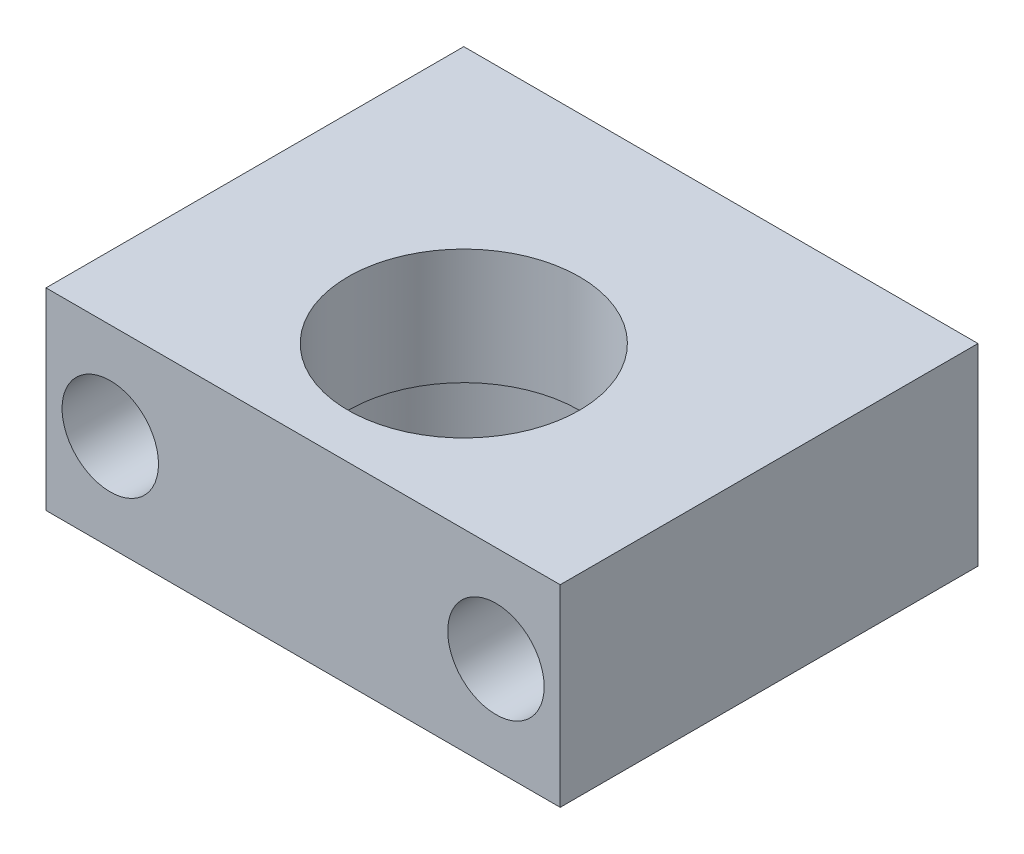
SolidWorks part; units mm, degrees
material "A6061"
ref_plane "前基準面" through (0, 0, 0) normal (0, 0, 1) x (1, 0, 0)
ref_plane "上基準面" through (0, 0, 0) normal (0, 1, 0) x (1, 0, 0)
ref_plane "右基準面" through (0, 0, 0) normal (1, 0, 0) x (0, 0, -1)
sketch "草图1" plane through (0, 0, 0) normal (0, 1, 0) x (1, 0, 0)
  line L1 (-225, -32.5) -> (225, -32.5)
  line L2 (-225, -32.5) -> (-225, 32.5)
  line L3 (-225, 32.5) -> (225, 32.5)
  line L4 (225, -32.5) -> (225, 32.5)
  line L5 (-225, -32.5) -> (225, 32.5) construction
  line L6 (-225, 32.5) -> (225, -32.5) construction
  point P0 (0, 0)
  dimension "D1" = 450
  dimension "D2" = 65
extrude "凸台-拉伸1" add sketch "草图1" along normal mid plane 30
chamfer "倒角1" distance 2 angle 45 2 edges at (225, 0, 32.5) (-225, 0, 32.5)
sketch "草图2" plane through (0, 15, 0) normal (0, 1, 0) x (1, 0, 0)
  line L0 (0, 83.4721) -> (0, 0) construction
  circle A0 centre (-200, 0) radius 10
  circle A1 centre (200, 0) radius 10
  dimension "D1" = 20
  dimension "D2" = 400
extrude "切除-拉伸1" cut sketch "草图2" against normal up to surface (30 mm away) up to face at (0, -15, 10.1667)
sketch "草图3" plane through (0, 15, 0) normal (0, 1, 0) x (1, 0, 0)
  line L0 (-225, 0) -> (-182, 0) construction
  line L2 (-225, 1) -> (-182, 1)
  line L3 (-225, -1) -> (-182, -1)
  line L4 (0, 108.9264) -> (0, 0) construction
  line L5 (225, 0) -> (182, 0) construction
  line L6 (225, 1) -> (182, 1)
  line L7 (225, -1) -> (182, -1)
  line L8 (-225, 32.5) -> (-225, -30.5) construction
  arc A0 (-225, 1) -> (-225, -1) centre (-225, 0) ccw
  arc A1 (-182, -1) -> (-182, 1) centre (-182, 0) ccw
  circle A2 centre (-200, 0) radius 10 construction
  arc A3 (225, 1) -> (225, -1) centre (225, 0) cw
  arc A4 (182, -1) -> (182, 1) centre (182, 0) cw
  point P2 (-200, 0)
  point P4 (-203.5, 0)
  point P16 (203.5, 0)
  dimension "D1" = 18
  dimension "D2" = 2
extrude "切除-拉伸2" cut sketch "草图3" against normal up to surface (30 mm away) up to face at (-200, -15, -10)
sketch "草图4" plane through (0, -15, 0) normal (0, 1, 0) x (1, 0, 0)
  line L0 (0, 70.3948) -> (0, 0) construction
  line L1 (225, 32.5) -> (-225, 32.5) construction
  circle A0 centre (0, -7.5) radius 21
  dimension "D1" = 42
  dimension "D2" = 40
extrude "切除-拉伸3" cut sketch "草图4" along normal blind 12
sketch "草图5" plane through (0, -3, 0) normal (0, -1, 0) x (-1, 0, 0)
  circle A0 centre (0, -7.5) radius 18
  circle A2 centre (0, -7.5) radius 21 construction
  dimension "D1" = 3
extrude "切除-拉伸4" cut sketch "草图5" against normal through all
hole_wizard "打孔尺寸(%根据)内六角圆柱头螺钉的类型2" positions "草图6" profile "草图7" counterbore size "M6" standard "GB"
sketch "草图6" plane through (0, 0, 32.5) normal (0, 0, 1) x (1, 0, 0)
  line L0 (0, -48.1525) -> (0, 0) construction
  line L1 (0, 0) -> (282.9731, 0) construction
  line L3 (225, 15) -> (225, -15) construction
  point P0 (215, -7.5)
  point P11 (215, 7.5)
  point P12 (-215, 7.5)
  point P13 (-215, -7.5)
  dimension "D1" = 15
  dimension "D2" = 10
sketch "草图7" plane through (215, -7.5, 32.5) normal (1, 0, 0) x (0, -1, 0)
  line L0 (0, 0) -> (0, 31.5)
  line L1 (0, 31.5) -> (3.3, 31.5)
  line L3 (3.3, 31.5) -> (3.3, 6.8)
  line L4 (3.3, 6.8) -> (5.5, 6.8)
  line L5 (5.5, 6.8) -> (5.5, 0)
  line L7 (5.5, 0) -> (0, 0)
  line L11 (0, -6.35) -> (0, 107.95) construction
  dimension "通孔孔直径" = 6.6
  dimension "通孔孔深度" = 31.5
  dimension "柱形沉头孔直径" = 11
  dimension "柱形沉头孔深度" = 6.8
hole_wizard "M6 螺纹孔1" positions "草图8" profile "草图9" tap size "M6" standard "GB" end condition through all
sketch "草图8" plane through (0, 0, -1) normal (0, 0, 1) x (1, 0, 0)
  point P0 (215, -7.5)
  point P3 (215, 7.5)
  point P6 (-215, -7.5)
  point P9 (-215, 7.5)
sketch "草图9" plane through (215, -7.5, -1) normal (1, 0, 0) x (0, -1, 0)
  line L0 (0, 0) -> (0, 31.5)
  line L1 (0, 31.5) -> (2.5, 31.5)
  line L2 (2.5, 31.5) -> (2.5, 0)
  line L5 (2.5, 0) -> (0, 0)
  line L11 (0, -6.35) -> (0, 107.95) construction
  dimension "通孔螺纹孔钻头直径" = 5
  dimension "通孔螺纹孔钻头深度" = 31.5
cosmetic thread "孔螺蚊线1" parameters "D2"=6
cosmetic thread "孔螺蚊线2" parameters "D2"=6
cosmetic thread "孔螺蚊线3" parameters "D2"=6
cosmetic thread "孔螺蚊线4" parameters "D2"=6
hole_wizard "打孔尺寸(%根据)内六角圆柱头螺钉的类型2" positions "草图10" profile "草图11" counterbore size "M8" standard "GB" end condition through all
sketch "草图10" plane through (0, 0, 32.5) normal (0, 0, 1) x (1, 0, 0)
  line L0 (0, -47.7503) -> (0, 0) construction
  point P0 (150, 0)
  point P2 (30, 0)
  point P10 (-30, 0)
  point P11 (-150, 0)
  dimension "D1" = 60
  dimension "D2" = 120
sketch "草图11" plane through (150, 0, 32.5) normal (1, 0, 0) x (0, -1, 0)
  line L0 (0, 0) -> (0, 65)
  line L1 (0, 65) -> (4.5, 65)
  line L3 (4.5, 65) -> (4.5, 55)
  line L4 (4.5, 55) -> (7.5, 55)
  line L5 (7.5, 55) -> (7.5, 0)
  line L7 (7.5, 0) -> (0, 0)
  line L11 (0, -6.35) -> (0, 107.95) construction
  dimension "通孔孔直径" = 9
  dimension "通孔孔深度" = 65
  dimension "柱形沉头孔直径" = 15
  dimension "柱形沉头孔深度" = 55
hole_wizard "M5 螺纹孔1" positions "草图12" profile "草图13" tap size "M5" standard "GB"
sketch "草图12" plane through (0, -15, 0) normal (0, -1, 0) x (-1, 0, 0)
  line L0 (0, 26.5553) -> (0, -7.5) construction
  circle A0 centre (0, -7.5) radius 24.5 construction
  point P0 (-17.3241, 9.8241)
  point P15 (17.3241, 9.8241)
  point P16 (17.3241, -24.8241)
  point P17 (-17.3241, -24.8241)
  dimension "D2" = 49
  dimension "D1" = 4
sketch "草图13" plane through (17.3241, -15, -9.8241) normal (1, 0, 0) x (0, 0, -1)
  line L0 (0, 0) -> (0, 13.6618)
  line L1 (0, 13.6618) -> (2.1, 12.4)
  line L2 (2.1, 12.4) -> (2.1, 0)
  line L5 (2.1, 0) -> (0, 0)
  line L10 (0, 13.6618) -> (-2.1, 12.4) construction
  line L11 (0, -6.35) -> (0, 107.95) construction
  dimension "螺纹孔钻头直径" = 4.2
  dimension "螺纹孔钻头深度" = 12.4
  dimension "导头角度" = 118
cosmetic thread "孔螺蚊线5" parameters "D1"=10, "D2"=5
cosmetic thread "孔螺蚊线6" parameters "D1"=10, "D2"=5
cosmetic thread "孔螺蚊线7" parameters "D1"=10, "D2"=5
cosmetic thread "孔螺蚊线8" parameters "D1"=10, "D2"=5
sketch "草图15" plane through (0, -15, 0) normal (0, -1, 0) x (1, 0, 0)
  line L0 (0, 5) -> (0, -66.1637) construction
  line L1 (277.4375, -66.1637) -> (40, -66.1637)
  line L2 (277.4375, -66.1637) -> (277.4375, 93.6551)
  line L3 (277.4375, 93.6551) -> (40, 93.6551)
  line L4 (40, -66.1637) -> (40, 93.6551)
  line L5 (-40, -66.1637) -> (-40, 93.6551)
  line L6 (-277.4375, 93.6551) -> (-40, 93.6551)
  line L7 (-277.4375, -66.1637) -> (-277.4375, 93.6551)
  line L8 (-277.4375, -66.1637) -> (-40, -66.1637)
  dimension "D1" = 80
extrude "切除-拉伸6" cut sketch "草图15" against normal through all
